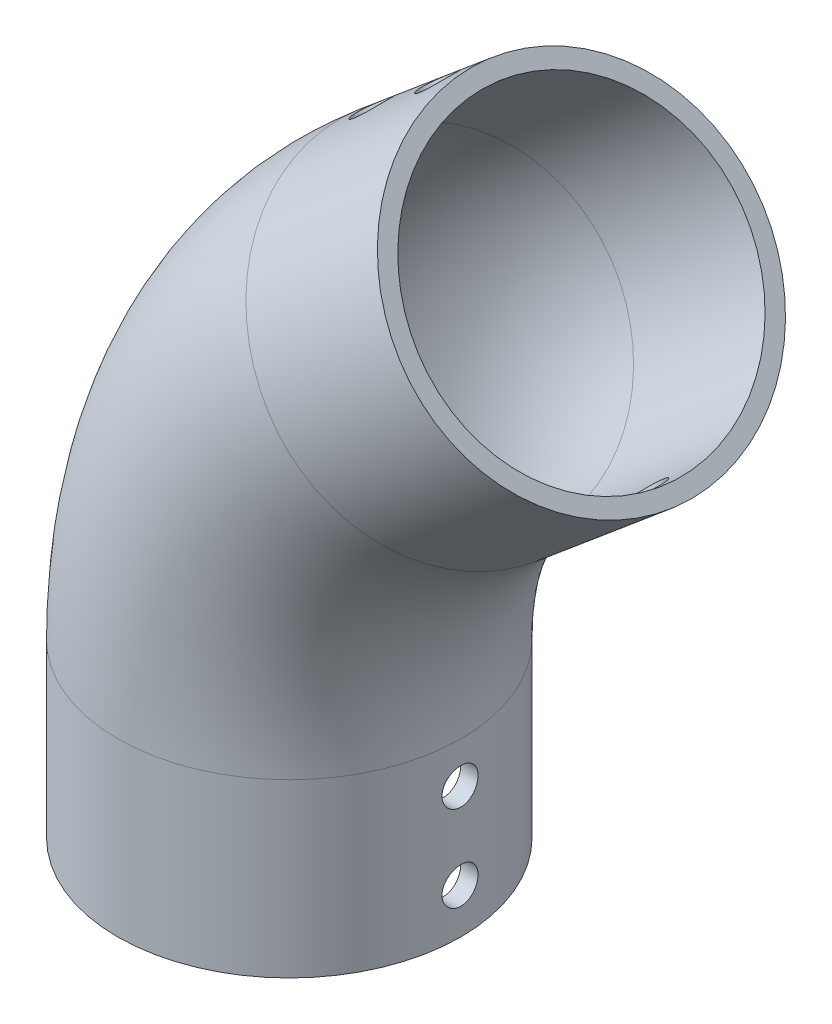
SolidWorks part; units mm, degrees
material "201 退火不锈钢 (SS)"
ref_plane "Z" through (0, 0, 0) normal (0, 0, 1) x (1, 0, 0)
ref_plane "上视基准面" through (0, 0, 0) normal (0, 1, 0) x (1, 0, 0)
ref_plane "右视基准面" through (0, 0, 0) normal (1, 0, 0) x (0, 0, -1)
sketch "草图1" plane through (0, 0, 0) normal (0, 0, 1) x (1, 0, 0)
  line L0 (0, 0) -> (0, 50)
  line L1 (46.7948, 150.3518) -> (85.097, 182.4912)
  arc A0 (46.7948, 150.3518) -> (0, 50) centre (131, 50) ccw
  dimension "D2" = 50
  dimension "D4" = 131
  dimension "D1" = 130
  dimension "D3" = 50
sketch "草图3" plane through (0, 0, 0) normal (0, 1, 0) x (1, 0, 0)
  circle A0 centre (0, 0) radius 50
  circle A1 centre (0, 0) radius 45
  dimension "D1" = 100
  dimension "D2" = 5
sweep "扫描2" add profiles "草图3" path "草图1"
sketch "草图4" plane through (0, 0, 0) normal (1, 0, 0) x (0, 0, -1)
  line L0 (0, 0) -> (0, 13) construction
  line L1 (0, 38) -> (0, 13) construction
  circle A6 centre (0, 13) radius 5.25
  circle A7 centre (0, 38) radius 5.25
  dimension "D2" = 10.5
  dimension "D1" = 13
  dimension "D3" = 25
extrude "切除-拉伸1" cut sketch "草图4" against normal mid plane 110
ref_plane "基准面1" through (42.5485, 91.2456, 0) normal (0.4226, 0.9063, 0) x (0.9063, -0.4226, 0)
mirror "镜向1" about plane through (42.5485, 91.2456, 0) normal (0.4226, 0.9063, 0) of "切除-拉伸1"
